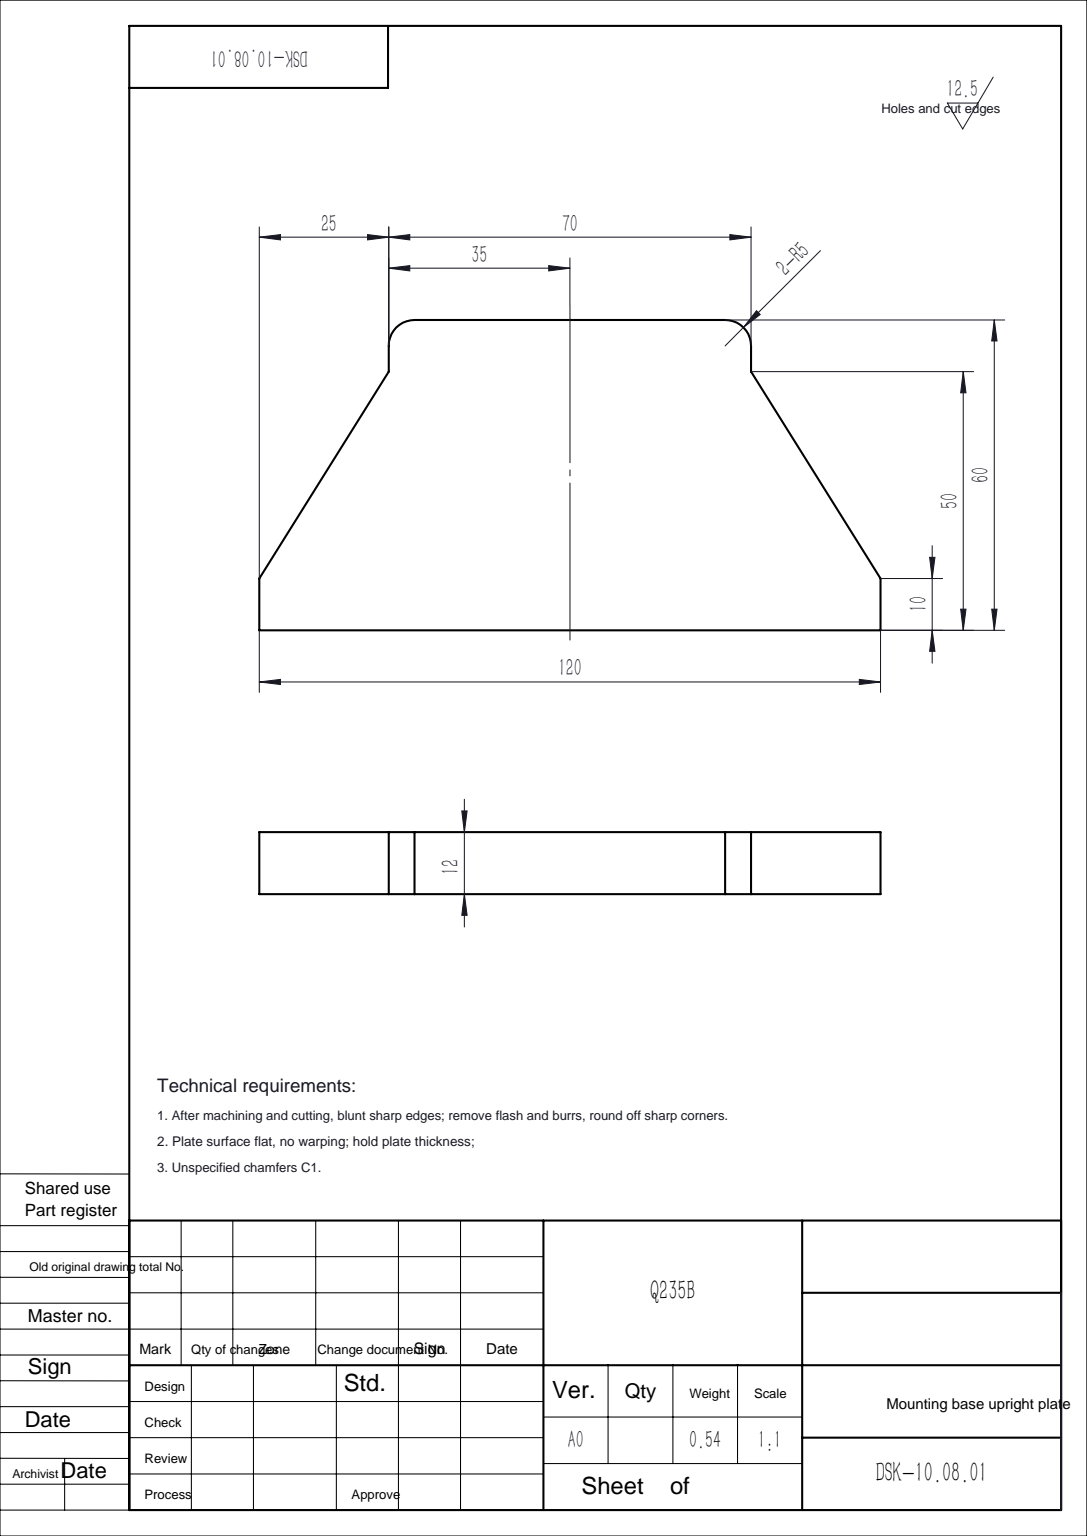
SolidWorks part; units mm, degrees
material "Q235B"
ref_plane "Front Plane" through (0, 0, 0) normal (0, 0, 1) x (1, 0, 0)
ref_plane "Top Plane" through (0, 0, 0) normal (0, 1, 0) x (1, 0, 0)
ref_plane "Right Plane" through (0, 0, 0) normal (1, 0, 0) x (0, 0, -1)
sketch "Sketch1" plane through (0, 0, 0) normal (0, 0, 1) x (1, 0, 0)
  line L0 (-60, 0) -> (60, 0)
  line L1 (60, 0) -> (60, 10)
  line L2 (60, 10) -> (35, 50)
  line L3 (35, 50) -> (35, 60)
  line L4 (35, 60) -> (-35, 60)
  line L5 (0, 60) -> (0, 0) construction
  line L6 (-35, 50) -> (-35, 60)
  line L7 (-60, 10) -> (-35, 50)
  line L8 (-60, 0) -> (-60, 10)
  dimension "D1" = 120
  dimension "D2" = 70
  dimension "D3" = 60
  dimension "D4" = 50
  dimension "D5" = 10
extrude "Boss-Extrude1" add sketch "Sketch1" along normal mid plane 12
fillet "Fillet1" radius 5 2 edges at (35, 60, 0) (-35, 60, 0)
